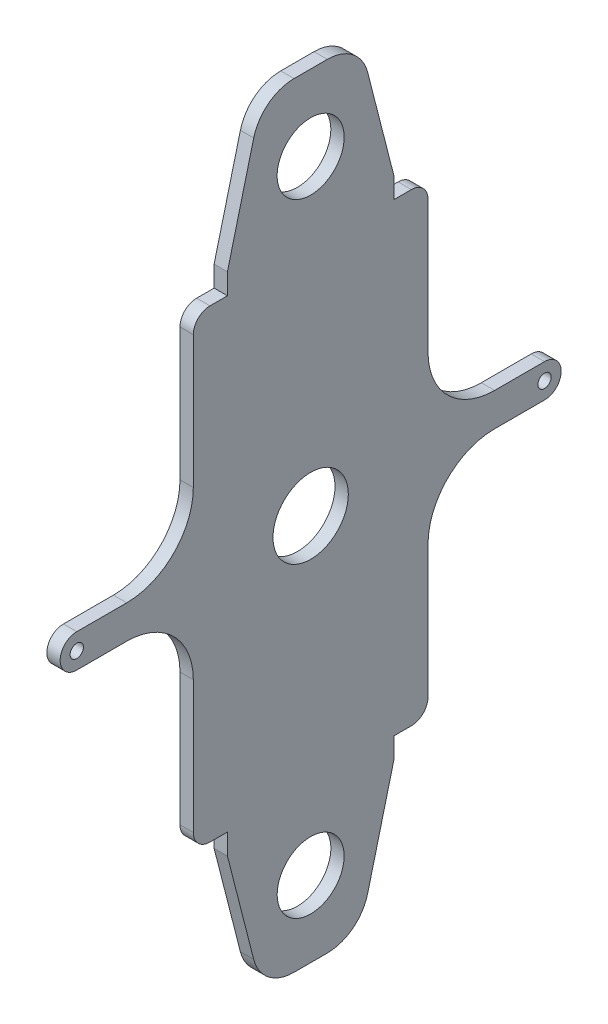
from build123d import *

# Parameters (mm, degrees)
SKETCH1_R           = 40.25
SKETCH1_R_2         = 45.25
SKETCH1_R_3         = 4.25
SKETCH1_R_4         = 3.5
SKETCH1_R_5         = 8
BOSS_EXTRUDE1_DEPTH = 16
FILLET1_R           = 20
SKETCH2_R           = 4.25
SKETCH2_R_2         = 3.5
BOSS_EXTRUDE2_DEPTH = 16


with BuildPart() as part:
    # Sketch1 → Boss-Extrude1 (new body)
    with BuildSketch(Plane(origin=(0, 0, 0), x_dir=(0, 0, -1), z_dir=(1, 0, 0))):
        with BuildLine():
            Line((-281, 20), (-221, 20))
            ThreePointArc((-221, 20), (-164.431457505, 43.431457505), (-141, 100))
            Line((-141, 100), (-141, 279))
            Line((-141, 279), (-100, 279))
            Line((-100, 279), (-100, 304))
            Line((-100, 304), (-68.44064835, 427.389656469))
            ThreePointArc((-68.44064835, 427.389656469), (-50.663636253, 454.493561649), (-20, 465))
            Line((-20, 465), (20, 465))
            ThreePointArc((20, 465), (50.663636253, 454.493561649), (68.44064835, 427.389656469))
            Line((68.44064835, 427.389656469), (100, 304))
            Line((100, 304), (100, 279))
            Line((100, 279), (141, 279))
            Line((141, 279), (141, 100))
            ThreePointArc((141, 100), (164.431457505, 43.431457505), (221, 20))
            Line((221, 20), (281, 20))
            ThreePointArc((281, 20), (301, 0), (281, -20))
            Line((281, -20), (221, -20))
            ThreePointArc((221, -20), (164.431457505, -43.431457505), (141, -100))
            Line((141, -100), (141, -279))
            Line((141, -279), (100, -279))
            Line((100, -279), (100, -304))
            Line((100, -304), (68.44064835, -427.389656469))
            ThreePointArc((68.44064835, -427.389656469), (50.663636253, -454.493561649), (20, -465))
            Line((20, -465), (-20, -465))
            ThreePointArc((-20, -465), (-50.663636253, -454.493561649), (-68.44064835, -427.389656469))
            Line((-68.44064835, -427.389656469), (-100, -304))
            Line((-100, -304), (-100, -279))
            Line((-100, -279), (-141, -279))
            Line((-141, -279), (-141, -100))
            ThreePointArc((-141, -100), (-164.431457505, -43.431457505), (-221, -20))
            Line((-221, -20), (-281, -20))
            ThreePointArc((-281, -20), (-301, 0), (-281, 20))
        make_face()
        with Locations((0, 374)):
            Circle(SKETCH1_R, mode=Mode.SUBTRACT)
        Circle(SKETCH1_R_2, mode=Mode.SUBTRACT)
        with Locations(Location((0, -374, 0), (0, 0, 180))):
            Circle(SKETCH1_R, mode=Mode.SUBTRACT)
        with Locations((20, -75)):
            Circle(SKETCH1_R_3, mode=Mode.SUBTRACT)
        with Locations((-20, -75)):
            Circle(SKETCH1_R_3, mode=Mode.SUBTRACT)
        with Locations((-20, 442)):
            Circle(SKETCH1_R_4, mode=Mode.SUBTRACT)
        with Locations((20, 442)):
            Circle(SKETCH1_R_4, mode=Mode.SUBTRACT)
        with Locations(Location((-20, -442, 0), (0, 0, 180))):
            Circle(SKETCH1_R_3, mode=Mode.SUBTRACT)
        with Locations(Location((20, -442, 0), (0, 0, 180))):
            Circle(SKETCH1_R_3, mode=Mode.SUBTRACT)
        with Locations((-281, 0)):
            Circle(SKETCH1_R_5, mode=Mode.SUBTRACT)
        with Locations((281, 0)):
            Circle(SKETCH1_R_5, mode=Mode.SUBTRACT)
    extrude(amount=BOSS_EXTRUDE1_DEPTH)

    # Fillet1
    fillet1_edges = [part.edges().sort_by_distance(p)[0] for p in [
        (8, 279, -141),
        (8, -279, -141),
        (8, -279, 141),
        (8, 279, 141),
    ]]
    fillet(fillet1_edges, radius=FILLET1_R)

    # Sketch2 → Boss-Extrude2 (add)
    with BuildSketch(Plane.ZY):
        with Locations((20, -442)):
            Circle(SKETCH2_R)
        with Locations((-20, -442)):
            Circle(SKETCH2_R)
        with Locations((20, -75)):
            Circle(SKETCH2_R)
        with Locations((-20, -75)):
            Circle(SKETCH2_R)
        with Locations((20, 442)):
            Circle(SKETCH2_R_2)
        with Locations((-20, 442)):
            Circle(SKETCH2_R_2)
    extrude(amount=-BOSS_EXTRUDE2_DEPTH)


solid = part.part
